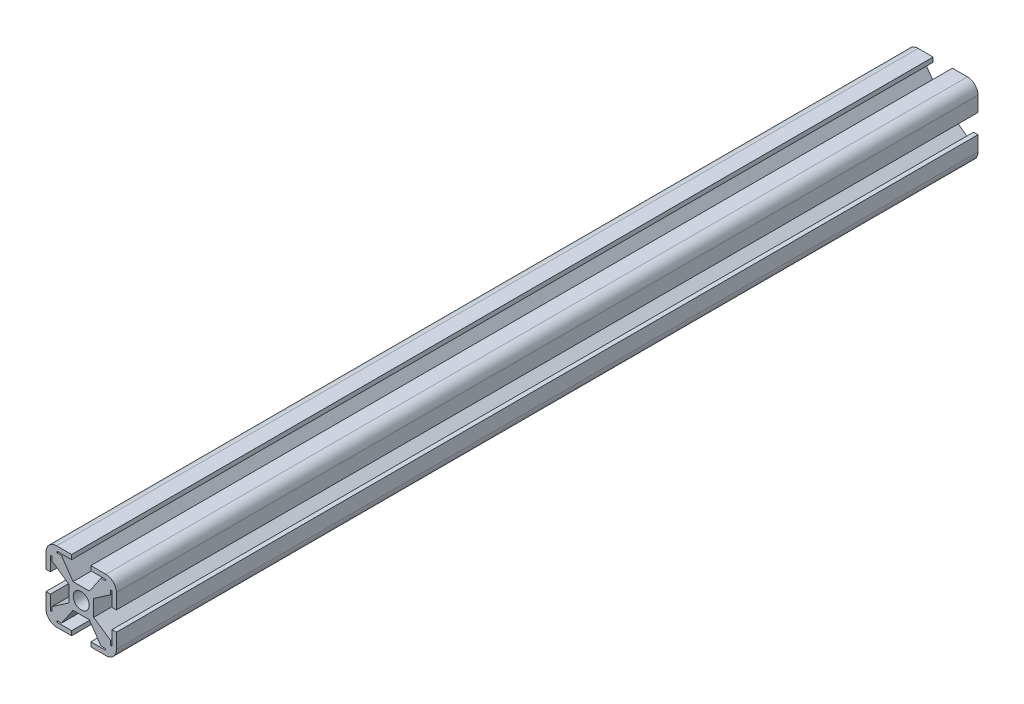
SolidWorks part; units mm, degrees
ref_plane "前视基准面" through (0, 0, 0) normal (0, 0, 1) x (1, 0, 0)
ref_plane "上视基准面" through (0, 0, 0) normal (0, 1, 0) x (1, 0, 0)
ref_plane "右视基准面" through (0, 0, 0) normal (1, 0, 0) x (0, 0, -1)
sketch "草图1" plane through (0, 0, 0) normal (0, 0, 1) x (1, 0, 0)
  line L1 (15, -15) -> (-15, -15)
  line L2 (15, -15) -> (15, 15)
  line L3 (15, 15) -> (-15, 15)
  line L4 (-15, -15) -> (-15, 15)
  line L5 (15, -15) -> (-15, 15) construction
  line L6 (15, 15) -> (-15, -15) construction
  point P0 (0, 0)
  dimension "D1" = 30
extrude "凸台-拉伸1" add sketch "草图1" along normal mid plane 367
fillet "圆角1" radius 4.5 4 edges at (15, -15, 0) (15, 15, 0) (-15, 15, 0) (-15, -15, 0)
sketch "草图2" plane through (0, 0, 183.5) normal (0, 0, 1) x (1, 0, 0)
  line L0 (10.5, 15) -> (-10.5, 15) construction
  line L1 (4.1, 17.2) -> (-4.1, 17.2)
  line L2 (4.1, 17.2) -> (4.1, 12.8)
  line L3 (4.1, 12.8) -> (-4.1, 12.8)
  line L4 (-4.1, 17.2) -> (-4.1, 12.8)
  line L5 (4.1, 17.2) -> (-4.1, 12.8) construction
  line L6 (4.1, 12.8) -> (-4.1, 17.2) construction
  line L7 (-10.25, 12.5) -> (-5.3, 5.3)
  line L8 (10.25, 13.1) -> (-10.25, 13.1)
  line L9 (10.25, 13.1) -> (10.25, 12.5)
  line L10 (10.25, 12.5) -> (-10.25, 12.5)
  line L11 (-10.25, 13.1) -> (-10.25, 12.5)
  line L12 (10.25, 13.1) -> (-10.25, 12.5) construction
  line L13 (10.25, 12.5) -> (-10.25, 13.1) construction
  line L14 (5.3, -5.3) -> (-5.3, -5.3)
  line L15 (5.3, -5.3) -> (5.3, 5.3)
  line L16 (5.3, 5.3) -> (-5.3, 5.3)
  line L17 (-5.3, -5.3) -> (-5.3, 5.3)
  line L18 (5.3, -5.3) -> (-5.3, 5.3) construction
  line L19 (5.3, 5.3) -> (-5.3, -5.3) construction
  line L20 (-8.4297, 12.5) -> (-3.4797, 5.3)
  line L21 (10.25, 12.5) -> (5.3, 5.3)
  line L22 (8.4297, 12.5) -> (3.4797, 5.3)
  circle A0 centre (0, 0) radius 3.4
  point P0 (0, 15)
  point P7 (0, 12.8)
  point P12 (0, 0)
  line M7 (10.5, 15) -> (-10.5, 15)
  dimension "D6" = 6.8
  dimension "D1" = 8.2
  dimension "D2" = 20.5
  dimension "D3" = 10.6
  dimension "D4" = 1.5
  dimension "D5" = 1.5
  dimension "D7" = 1.9
  dimension "D8" = 12.5
extrude "切除-拉伸1" cut sketch "草图2" against normal through all contours L2 L8 L4 L3 | L8 L2 L4 M7 | L8 L11 L10 L9 L2 L3 L4 | L22 L10 L20 L16 | A0
pattern_circular "阵列(圆周)1" count 4 over 360 about axis through (0, 0, 0) along (0, 0, 1) of "切除-拉伸1"
